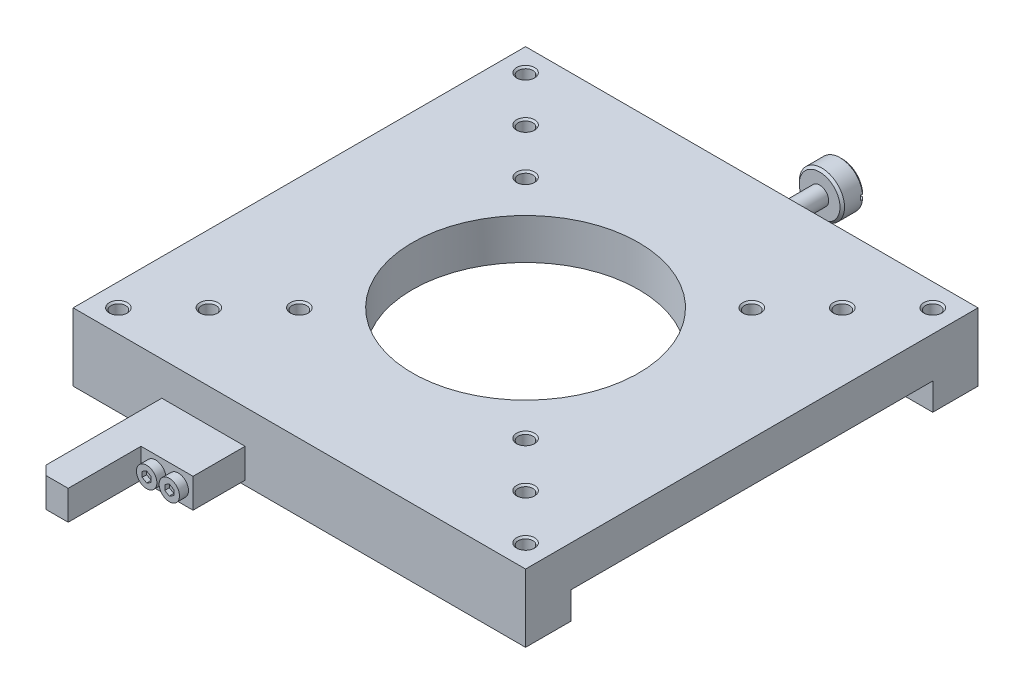
from build123d import *

# Parameters (mm, degrees)
EXTRUDE_1_DEPTH      = 50
EXTRUDE_1_DEPTH_BACK = 50
EXTRUDE_2_DEPTH      = 6.5
SKETCH_16_R          = 25
CUT_EXTRUDE_1_DEPTH  = 50
SKETCH_17_W          = 10
SKETCH_17_H          = 1
CUT_EXTRUDE_2_DEPTH  = 1
SKETCH_18_R          = 2.25
EXTRUDE_3_DEPTH      = 2
SKETCH_19_R          = 2.25
EXTRUDE_4_DEPTH      = 2
CUT_EXTRUDE_3_DEPTH  = 1
CUT_EXTRUDE_4_DEPTH  = 1


with BuildPart() as part:
    # 草图1 → 凸台-拉伸1 (new, two sides: drawn at the far end of the back side and taken through both)
    with BuildSketch(Plane(origin=(0, 0, 0), x_dir=(0, 0, -1), z_dir=(1, 0, 0)).offset(-EXTRUDE_1_DEPTH_BACK)):
        Polygon((-50, 15), (-50, 0), (-40, 0), (-40, 6), (40, 6), (40, 0), (50, 0), (50, 15), align=None)
    extrude(amount=EXTRUDE_1_DEPTH + EXTRUDE_1_DEPTH_BACK)

    # 草图2 → 旋转1 (revolve)
    with BuildSketch(Plane(origin=(0, 0, 0), x_dir=(0, 0, -1), z_dir=(1, 0, 0)), mode=Mode.PRIVATE) as revolve_1_sk:
        Polygon((50, 4), (50, 5), (50.75, 5), (50.75, 6), (65, 6), (65, 8.5), (65.5, 9), (69.5, 9), (70, 8.5), (70, 4), align=None)
    revolve(revolve_1_sk.sketch.rotate(Axis((0, 4, -70), (0, 0, 1)), 270), axis=Axis((0, 4, -70), (0, 0, 1)))

    # 草图3 → 凸台-拉伸2 (add)
    with BuildSketch(Plane(origin=(0, 7.5, 0), x_dir=(-1, 0, 0), z_dir=(0, 1, 0))):
        Polygon((30.4, 50), (30.4, 75.6), (28.4, 77.6), (23.5, 77.6), (23.5, 61.5), (12, 61.5), (12, 50), align=None)
    extrude(amount=-EXTRUDE_2_DEPTH)

    # 草图4 → 切除-旋转1 (revolve, cut)
    with BuildSketch(Plane.XY.offset(45), mode=Mode.PRIVATE) as cut_revolve_1_sk:
        Polygon((-45, 15), (-43, 15), (-43.379, 14.621), (-43.379, 8.135884786), (-45, 7.2), align=None)
    revolve(cut_revolve_1_sk.sketch.rotate(Axis((-45, 7.2, 45), (0, 1, 0)), 270), axis=Axis((-45, 7.2, 45), (0, 1, 0)), mode=Mode.SUBTRACT)

    # 草图5 → 切除-旋转2 (revolve, cut)
    with BuildSketch(Plane.XY.offset(45), mode=Mode.PRIVATE) as cut_revolve_2_sk:
        Polygon((45, 15), (47, 15), (46.621, 14.621), (46.621, 8.135884786), (45, 7.2), align=None)
    revolve(cut_revolve_2_sk.sketch.rotate(Axis((45, 7.2, 45), (0, 1, 0)), 270), axis=Axis((45, 7.2, 45), (0, 1, 0)), mode=Mode.SUBTRACT)

    # 草图6 → 切除-旋转3 (revolve, cut)
    with BuildSketch(Plane.XY.offset(-45), mode=Mode.PRIVATE) as cut_revolve_3_sk:
        Polygon((-45, 15), (-43, 15), (-43.379, 14.621), (-43.379, 8.135884786), (-45, 7.2), align=None)
    revolve(cut_revolve_3_sk.sketch.rotate(Axis((-45, 7.2, -45), (0, 1, 0)), 270), axis=Axis((-45, 7.2, -45), (0, 1, 0)), mode=Mode.SUBTRACT)

    # 草图7 → 切除-旋转4 (revolve, cut)
    with BuildSketch(Plane.XY.offset(-45), mode=Mode.PRIVATE) as cut_revolve_4_sk:
        Polygon((45, 15), (47, 15), (46.621, 14.621), (46.621, 8.135884786), (45, 7.2), align=None)
    revolve(cut_revolve_4_sk.sketch.rotate(Axis((45, 7.2, -45), (0, 1, 0)), 270), axis=Axis((45, 7.2, -45), (0, 1, 0)), mode=Mode.SUBTRACT)

    # 草图8 → 切除-旋转5 (revolve, cut)
    with BuildSketch(Plane.XY.offset(-35), mode=Mode.PRIVATE) as cut_revolve_5_sk:
        Polygon((35, 15), (37, 15), (36.621, 14.621), (36.621, 8.135884786), (35, 7.2), align=None)
    revolve(cut_revolve_5_sk.sketch.rotate(Axis((35, 7.2, -35), (0, 1, 0)), 270), axis=Axis((35, 7.2, -35), (0, 1, 0)), mode=Mode.SUBTRACT)

    # 草图9 → 切除-旋转6 (revolve, cut)
    with BuildSketch(Plane.XY.offset(-35), mode=Mode.PRIVATE) as cut_revolve_6_sk:
        Polygon((-35, 15), (-33, 15), (-33.379, 14.621), (-33.379, 8.135884786), (-35, 7.2), align=None)
    revolve(cut_revolve_6_sk.sketch.rotate(Axis((-35, 7.2, -35), (0, 1, 0)), 270), axis=Axis((-35, 7.2, -35), (0, 1, 0)), mode=Mode.SUBTRACT)

    # 草图10 → 切除-旋转7 (revolve, cut)
    with BuildSketch(Plane.XY.offset(35), mode=Mode.PRIVATE) as cut_revolve_7_sk:
        Polygon((-35, 15), (-33, 15), (-33.379, 14.621), (-33.379, 8.135884786), (-35, 7.2), align=None)
    revolve(cut_revolve_7_sk.sketch.rotate(Axis((-35, 7.2, 35), (0, 1, 0)), 270), axis=Axis((-35, 7.2, 35), (0, 1, 0)), mode=Mode.SUBTRACT)

    # 草图11 → 切除-旋转8 (revolve, cut)
    with BuildSketch(Plane.XY.offset(35), mode=Mode.PRIVATE) as cut_revolve_8_sk:
        Polygon((35, 15), (37, 15), (36.621, 14.621), (36.621, 8.135884786), (35, 7.2), align=None)
    revolve(cut_revolve_8_sk.sketch.rotate(Axis((35, 7.2, 35), (0, 1, 0)), 270), axis=Axis((35, 7.2, 35), (0, 1, 0)), mode=Mode.SUBTRACT)

    # 草图12 → 切除-旋转9 (revolve, cut)
    with BuildSketch(Plane.XY.offset(-25), mode=Mode.PRIVATE) as cut_revolve_9_sk:
        Polygon((25, 15), (27, 15), (26.621, 14.621), (26.621, 8.135884786), (25, 7.2), align=None)
    revolve(cut_revolve_9_sk.sketch.rotate(Axis((25, 7.2, -25), (0, 1, 0)), 270), axis=Axis((25, 7.2, -25), (0, 1, 0)), mode=Mode.SUBTRACT)

    # 草图13 → 切除-旋转10 (revolve, cut)
    with BuildSketch(Plane.XY.offset(-25), mode=Mode.PRIVATE) as cut_revolve_10_sk:
        Polygon((-25, 15), (-23, 15), (-23.379, 14.621), (-23.379, 8.135884786), (-25, 7.2), align=None)
    revolve(cut_revolve_10_sk.sketch.rotate(Axis((-25, 7.2, -25), (0, 1, 0)), 270), axis=Axis((-25, 7.2, -25), (0, 1, 0)), mode=Mode.SUBTRACT)

    # 草图14 → 切除-旋转11 (revolve, cut)
    with BuildSketch(Plane.XY.offset(25), mode=Mode.PRIVATE) as cut_revolve_11_sk:
        Polygon((-25, 15), (-23, 15), (-23.379, 14.621), (-23.379, 8.135884786), (-25, 7.2), align=None)
    revolve(cut_revolve_11_sk.sketch.rotate(Axis((-25, 7.2, 25), (0, 1, 0)), 270), axis=Axis((-25, 7.2, 25), (0, 1, 0)), mode=Mode.SUBTRACT)

    # 草图15 → 切除-旋转12 (revolve, cut)
    with BuildSketch(Plane.XY.offset(25), mode=Mode.PRIVATE) as cut_revolve_12_sk:
        Polygon((25, 15), (27, 15), (26.621, 14.621), (26.621, 8.135884786), (25, 7.2), align=None)
    revolve(cut_revolve_12_sk.sketch.rotate(Axis((25, 7.2, 25), (0, 1, 0)), 270), axis=Axis((25, 7.2, 25), (0, 1, 0)), mode=Mode.SUBTRACT)

    # 草图16 → 切除-拉伸1 (cut)
    with BuildSketch(Plane(origin=(0, 0, 0), x_dir=(-1, 0, 0), z_dir=(0, 1, 0))):
        with Locations(Location((0, 0, 0), (0, 0, 270))):
            Circle(SKETCH_16_R)
    extrude(amount=CUT_EXTRUDE_1_DEPTH, mode=Mode.SUBTRACT)

    # 草图17 → 切除-拉伸2 (cut)
    with BuildSketch(Plane(origin=(0, 0, -70), x_dir=(-1, 0, 0), z_dir=(0, 0, -1))):
        with Locations((0, 4)):
            Rectangle(SKETCH_17_W, SKETCH_17_H)
    extrude(amount=-CUT_EXTRUDE_2_DEPTH, mode=Mode.SUBTRACT)

    # 草图18 → 凸台-拉伸3 (add)
    with BuildSketch(Plane.XY.offset(61.5)):
        with Locations((-20.25, 4.25)):
            Circle(SKETCH_18_R)
    extrude(amount=EXTRUDE_3_DEPTH)

    # 草图19 → 凸台-拉伸4 (add)
    with BuildSketch(Plane.XY.offset(61.5)):
        with Locations((-15.25, 4.25)):
            Circle(SKETCH_19_R)
    extrude(amount=EXTRUDE_4_DEPTH)

    # 草图20 → 切除-拉伸3 (cut)
    with BuildSketch(Plane.XY.offset(63.5)):
        Polygon((-16.25, 3.672649731), (-15.25, 3.095299462), (-14.25, 3.672649731), (-14.25, 4.827350269), (-15.25, 5.404700538), (-16.25, 4.827350269), align=None)
    extrude(amount=-CUT_EXTRUDE_3_DEPTH, mode=Mode.SUBTRACT)

    # 草图21 → 切除-拉伸4 (cut)
    with BuildSketch(Plane.XY.offset(63.5)):
        Polygon((-21.25, 3.672649731), (-20.25, 3.095299462), (-19.25, 3.672649731), (-19.25, 4.827350269), (-20.25, 5.404700538), (-21.25, 4.827350269), align=None)
    extrude(amount=-CUT_EXTRUDE_4_DEPTH, mode=Mode.SUBTRACT)


solid = part.part
